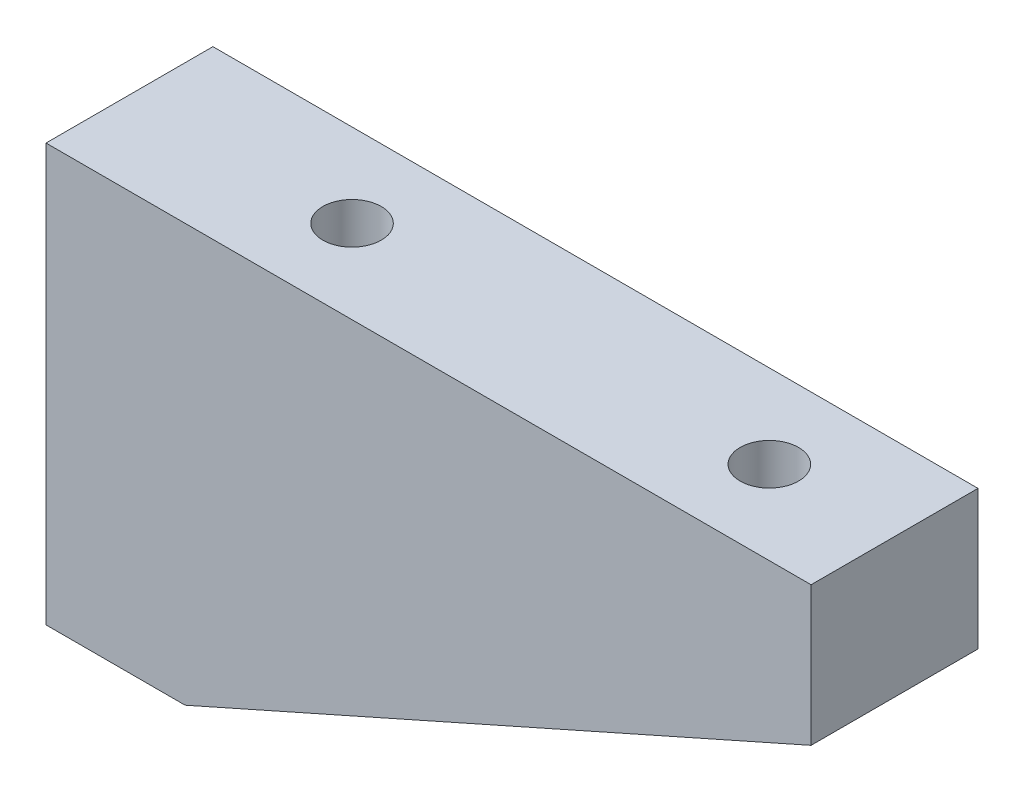
SolidWorks part; units mm, degrees
material "6061 合金"
ref_plane "前视基准面" through (0, 0, 0) normal (0, 0, 1) x (1, 0, 0)
ref_plane "上视基准面" through (0, 0, 0) normal (0, 1, 0) x (1, 0, 0)
ref_plane "右视基准面" through (0, 0, 0) normal (1, 0, 0) x (0, 0, -1)
sketch "草图1" plane through (0, 0, 0) normal (0, 0, 1) x (1, 0, 0)
  line L0 (-30.1067, 4.1186) -> (-40.1067, 4.1186)
  line L1 (-40.1067, 4.1186) -> (-40.1067, 34.1186)
  line L2 (-40.1067, 34.1186) -> (14.8933, 34.1186)
  line L3 (14.8933, 34.1186) -> (14.8933, 24.1186)
  line L4 (14.8933, 24.1186) -> (-30.1067, 4.1186)
  dimension "D1" = 55
  dimension "D2" = 10
  dimension "D3" = 10
  dimension "D4" = 30
extrude "凸台-拉伸1" add sketch "草图1" along normal blind 12
sketch "草图2" plane through (0, 34.1186, 0) normal (0, 1, 0) x (1, 0, 0)
  line L1 (5.8933, -12) -> (5.8933, 0) construction
  line L2 (-24.1067, -12) -> (-24.1067, 0)
  line L3 (-24.1067, -12) -> (-24.1067, 0) construction
  dimension "D1" = 16
  dimension "D2" = 30
hole_wizard "M5 螺纹孔1" positions "3D草图4" profile "草图6" tap size "M5" standard "GB"
sketch3d "3D草图4"
  line L0 (-24.1067, 34.1186, 12) -> (-24.1067, 34.1186, 0) construction
  line L1 (5.8933, 34.1186, 12) -> (5.8933, 34.1186, 0) construction
  point P0 (-24.1067, 34.1186, 6)
  point P4 (5.8933, 34.1186, 6)
  dimension "D1" = 30
  dimension "D2" = 6
sketch "草图6" plane through (-24.1067, 34.1186, 6) normal (1, 0, 0) x (0, 0, 1)
  line L0 (0, 0) -> (0, 11.2618)
  line L1 (0, 11.2618) -> (2.1, 10)
  line L2 (2.1, 10) -> (2.1, 0)
  line L5 (2.1, 0) -> (0, 0)
  line L10 (0, 11.2618) -> (-2.1, 10) construction
  line L11 (0, -6.35) -> (0, 107.95) construction
  dimension "螺纹孔钻头直径" = 4.2
  dimension "螺纹孔钻头深度" = 10
  dimension "导头角度" = 118
cosmetic thread "孔螺蚊线1" parameters "D1"=10, "D2"=5
cosmetic thread "孔螺蚊线2" parameters "D1"=10, "D2"=5
sketch "草图7" plane through (-40.1067, 0, 0) normal (-1, 0, 0) x (0, 0, 1)
  line L2 (12, 9.1186) -> (0, 9.1186)
  line L3 (12, 29.1186) -> (0, 29.1186)
  line L4 (12, 29.1186) -> (0, 29.1186)
  dimension "D1" = 5
  dimension "D2" = 20
hole_wizard "M5 螺纹孔2" positions "3D草图5" profile "草图8" tap size "M5" standard "GB"
sketch3d "3D草图5"
  line L0 (-40.1067, 9.1186, 12) -> (-40.1067, 9.1186, 0) construction
  line L1 (-40.1067, 29.1186, 12) -> (-40.1067, 29.1186, 0) construction
  point P0 (-40.1067, 9.1186, 6)
  point P4 (-40.1067, 29.1186, 6)
  dimension "D1" = 6
  dimension "D2" = 6
sketch "草图8" plane through (-40.1067, 9.1186, 6) normal (0, 1, 0) x (0, 0, 1)
  line L0 (0, 0) -> (0, 11.2618)
  line L1 (0, 11.2618) -> (2.1, 10)
  line L2 (2.1, 10) -> (2.1, 0)
  line L5 (2.1, 0) -> (0, 0)
  line L10 (0, 11.2618) -> (-2.1, 10) construction
  line L11 (0, -6.35) -> (0, 107.95) construction
  dimension "螺纹孔钻头直径" = 4.2
  dimension "螺纹孔钻头深度" = 10
  dimension "导头角度" = 118
cosmetic thread "孔螺蚊线3" parameters "D1"=10, "D2"=5
cosmetic thread "孔螺蚊线4" parameters "D1"=10, "D2"=5
